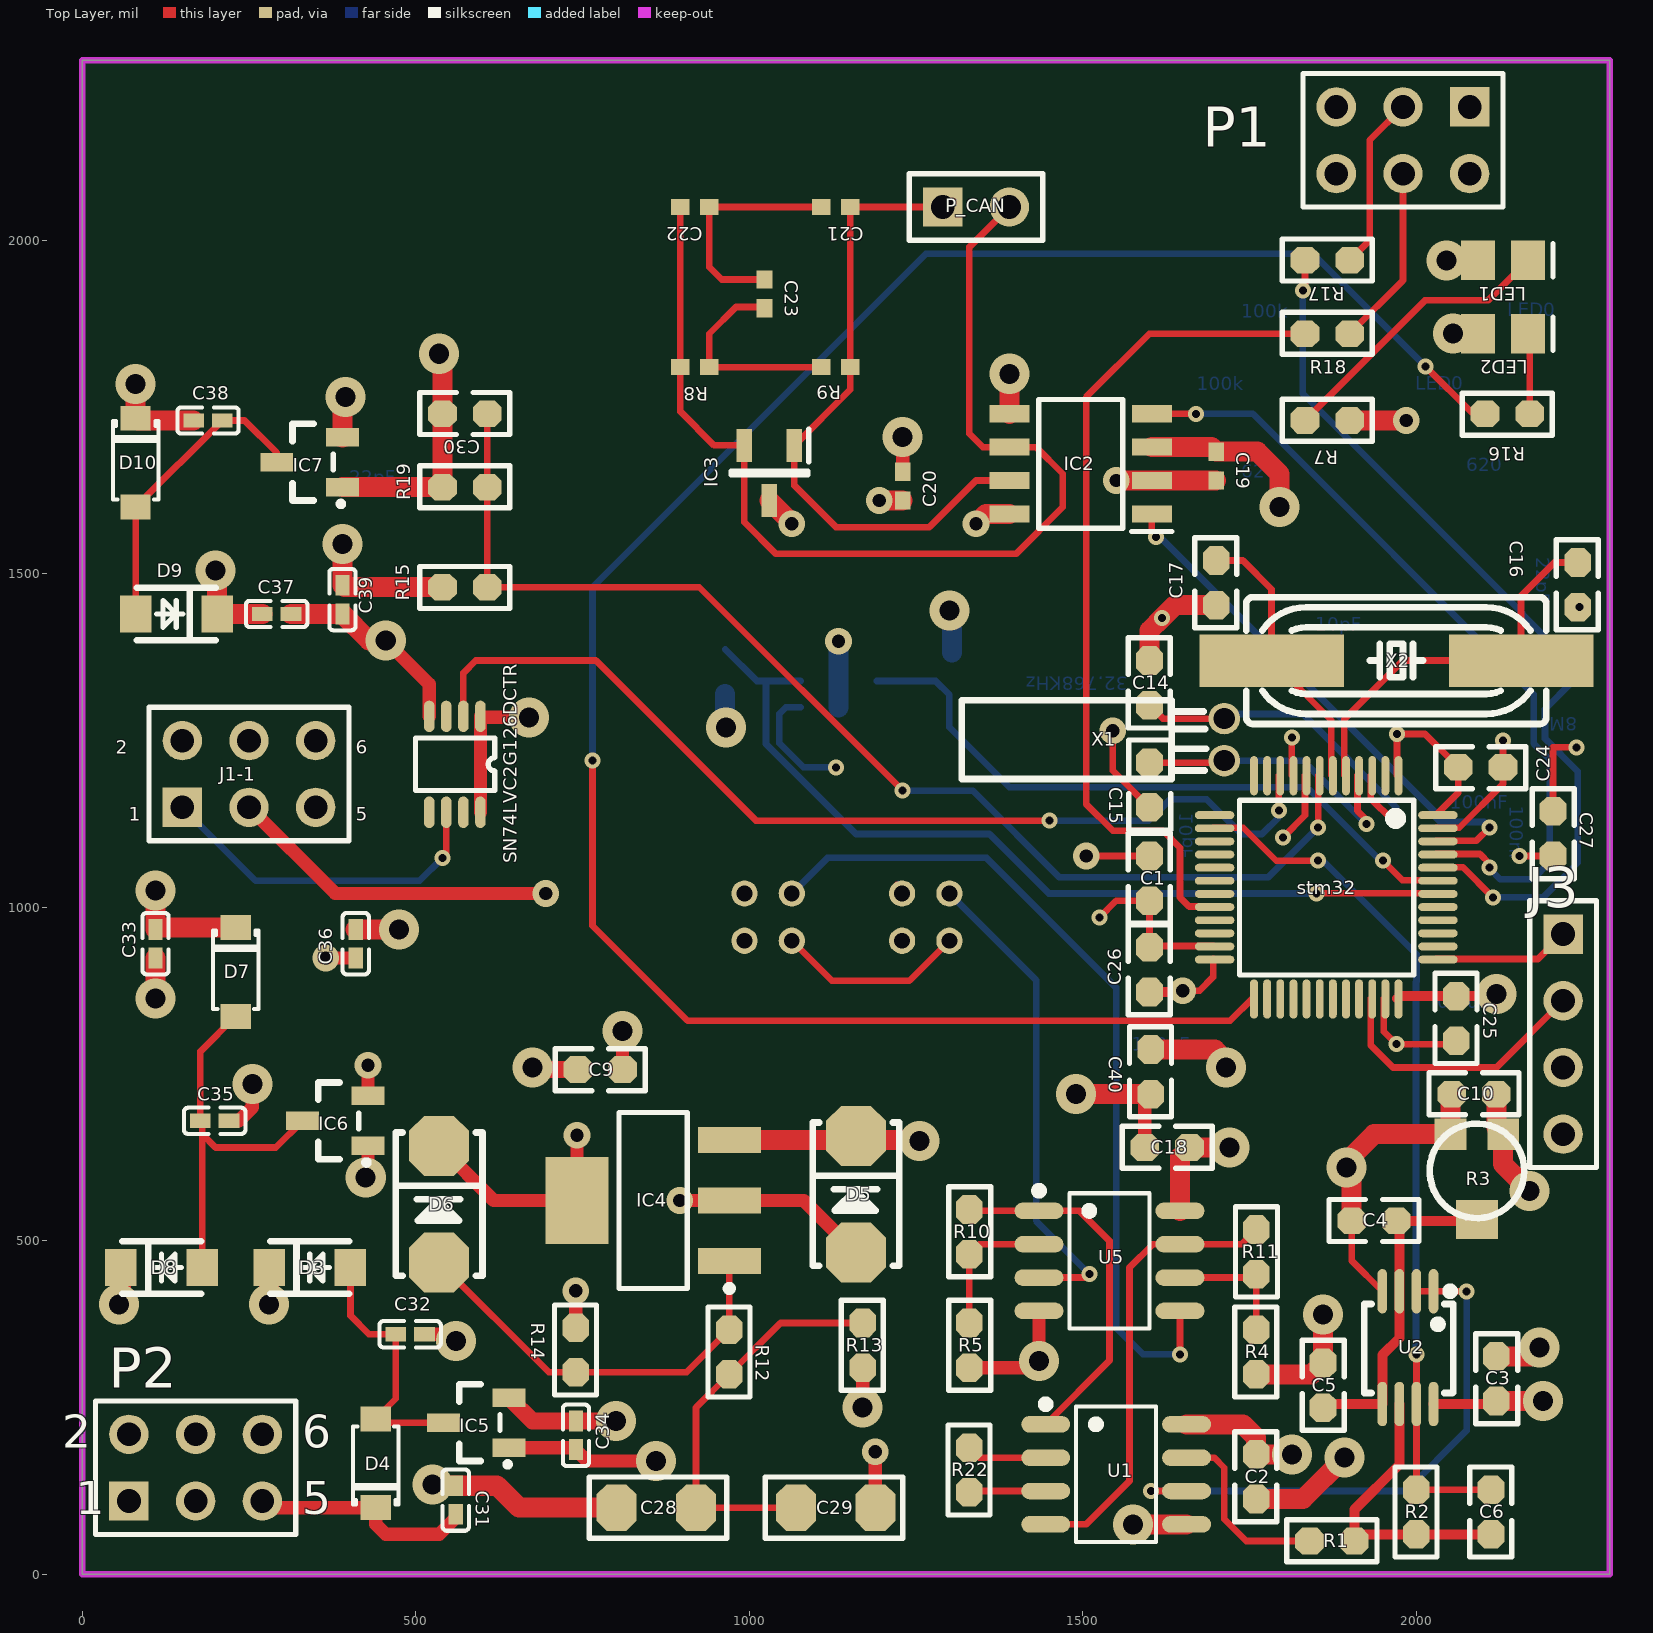
[diagram p0: Top Layer view]
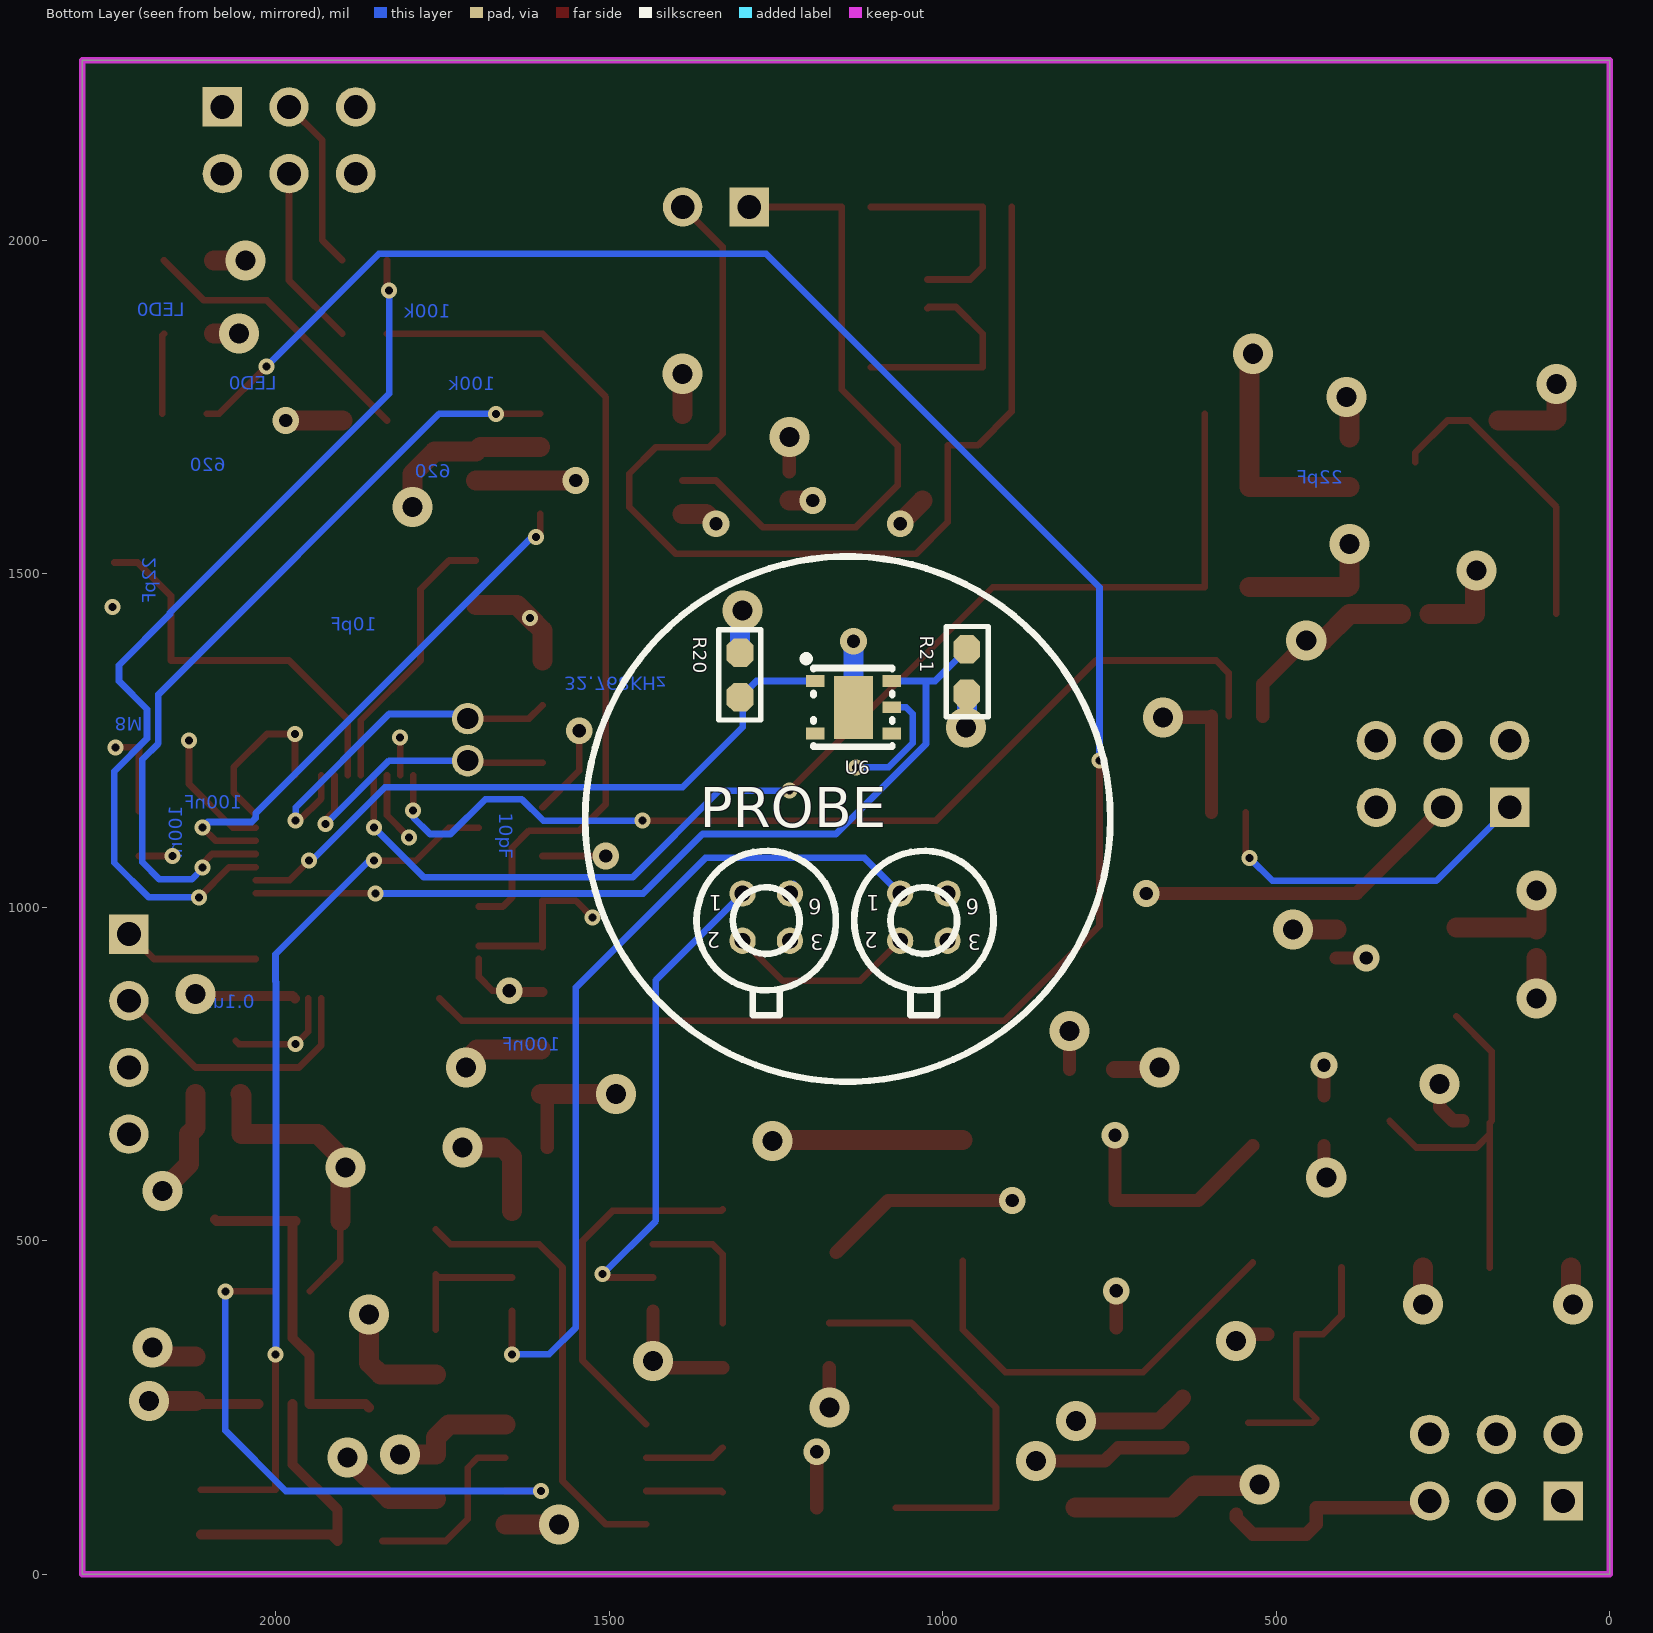
[diagram p1: Bottom Layer view, seen from below]
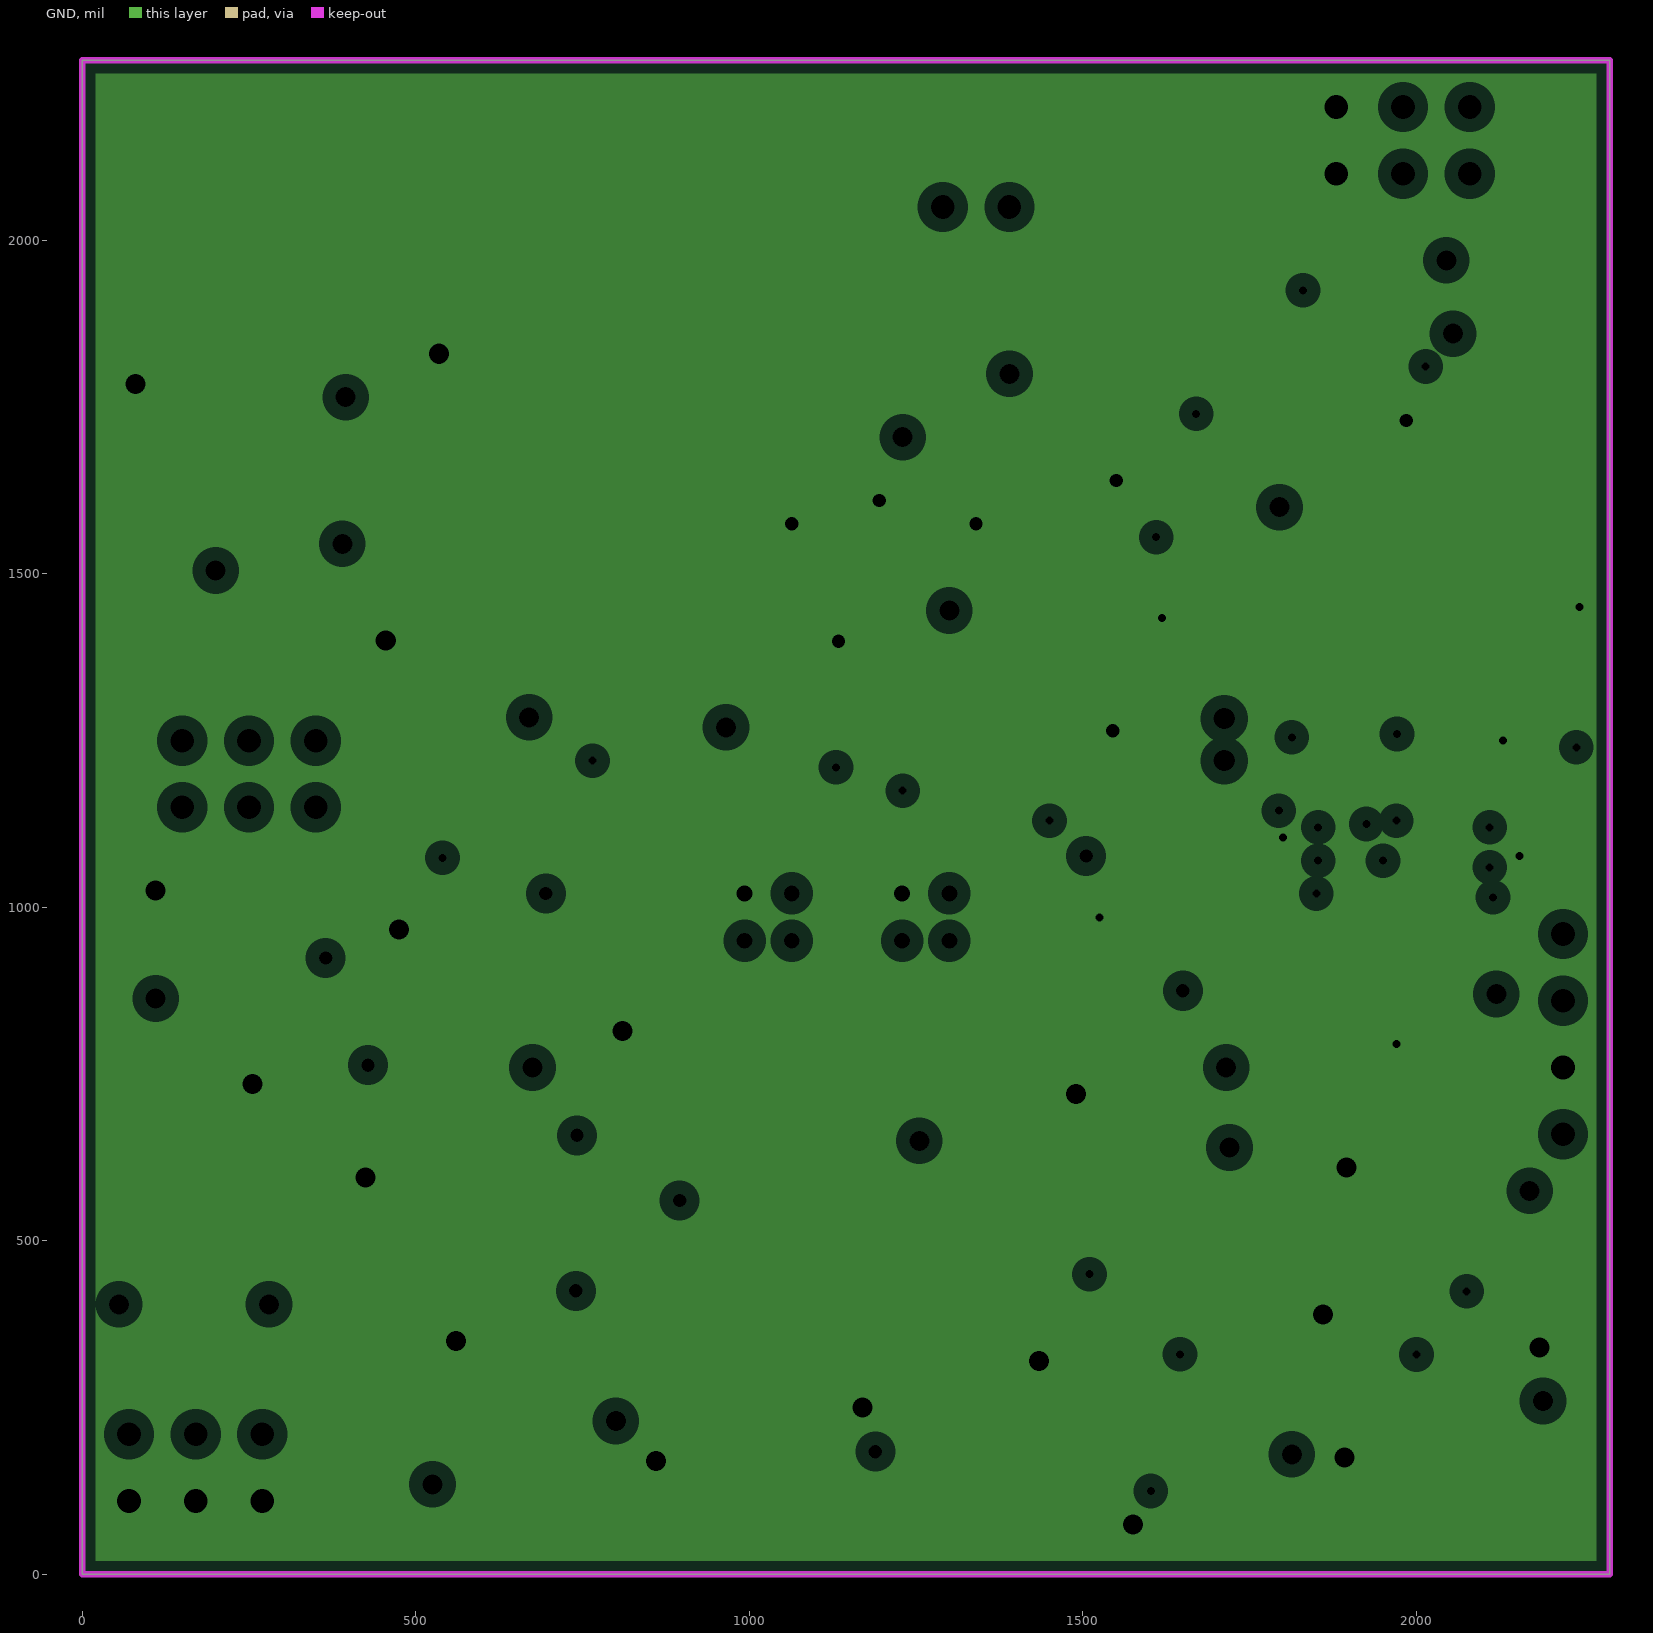
[diagram p2: GND, clearances drawn from the general rule]
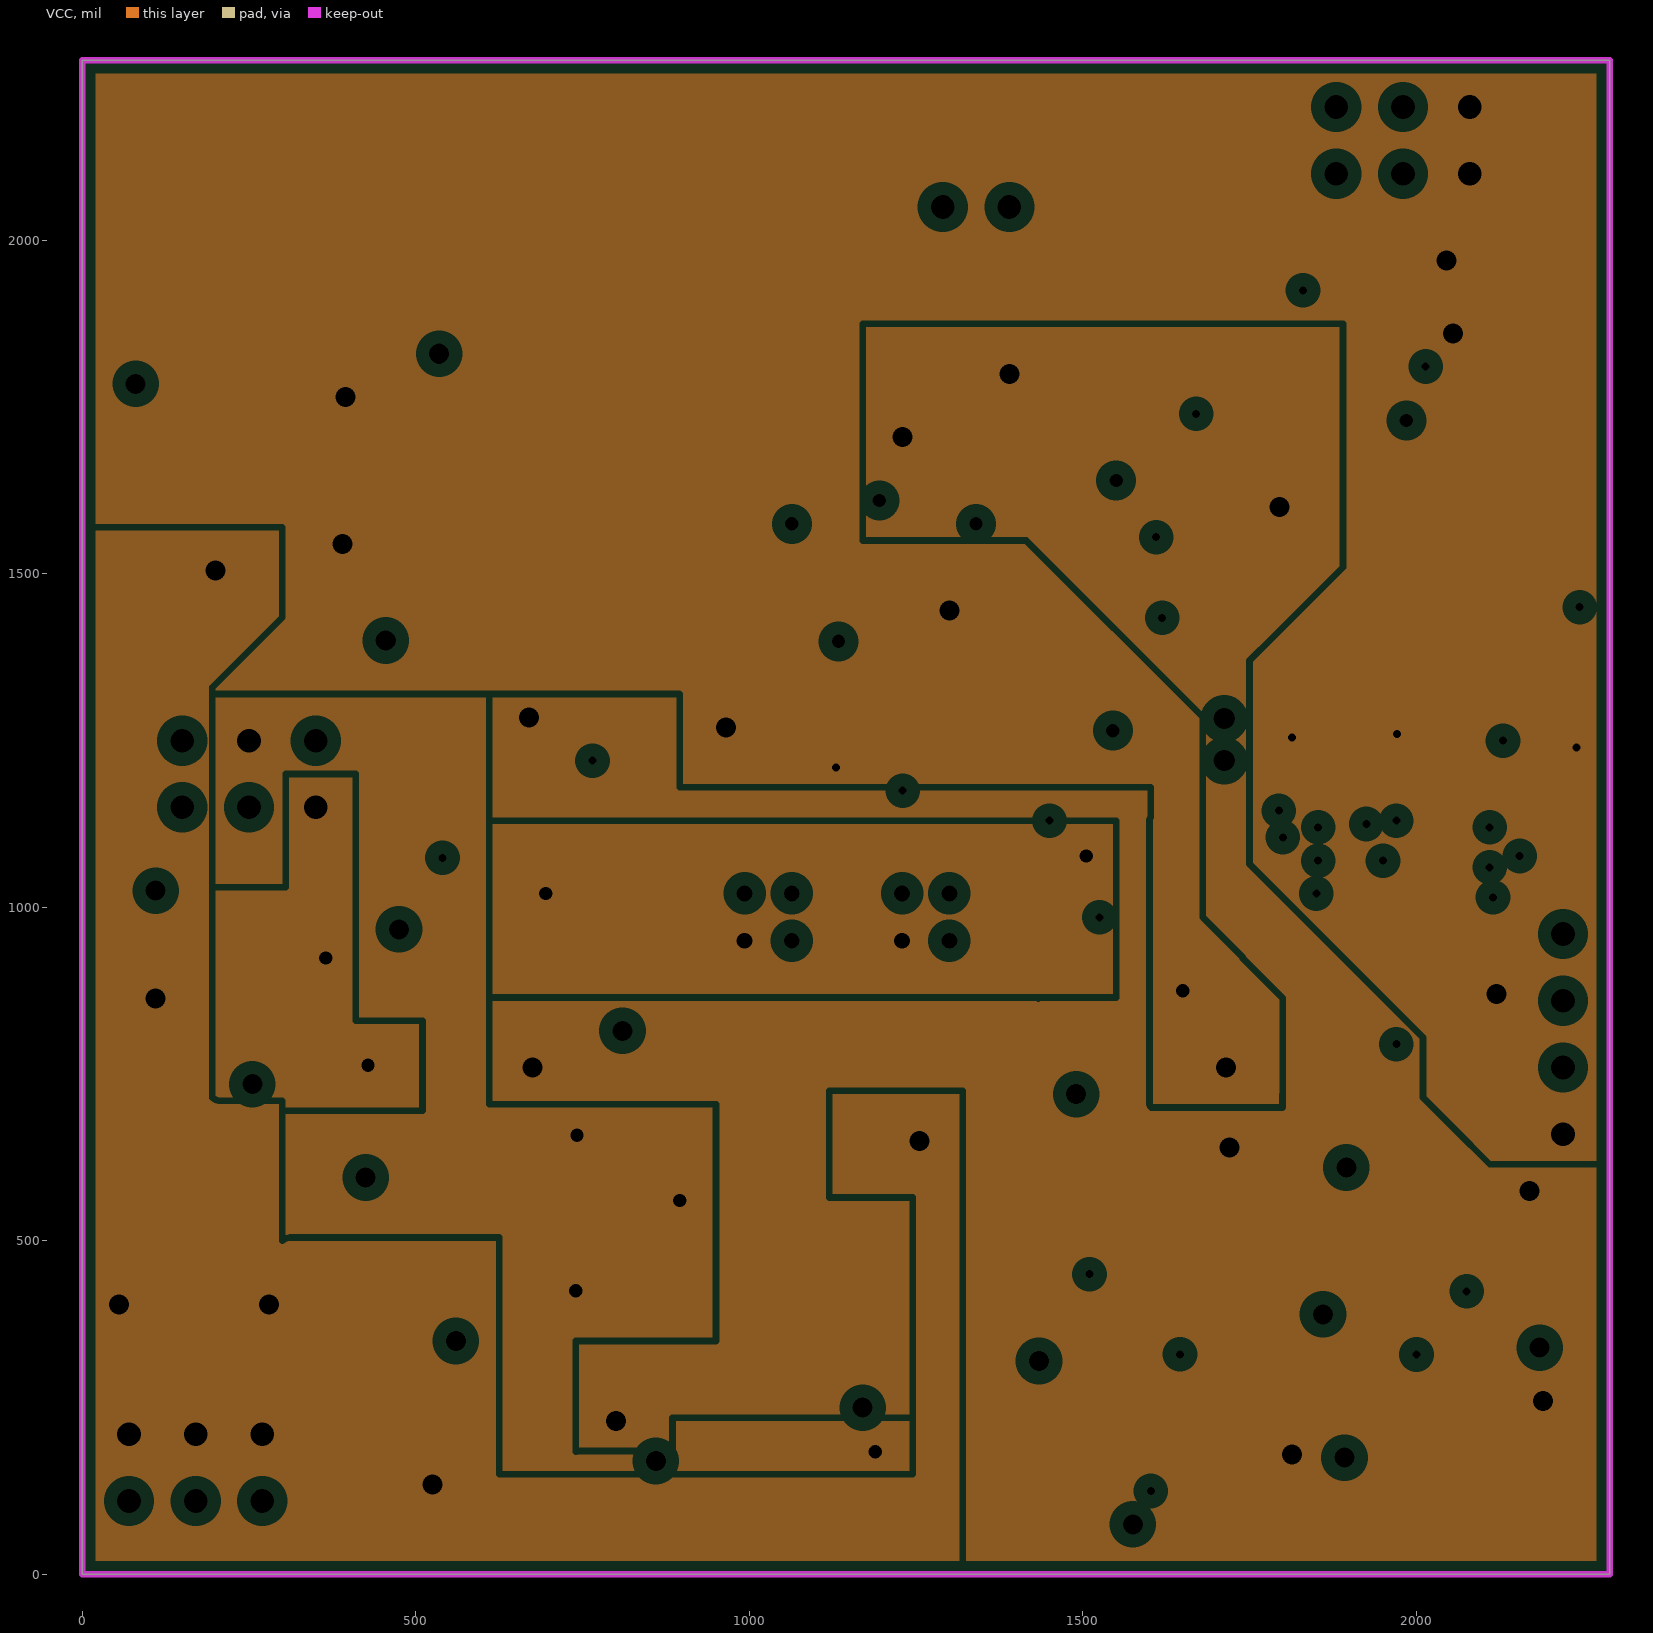
[diagram p3: VCC, clearances drawn from the general rule]
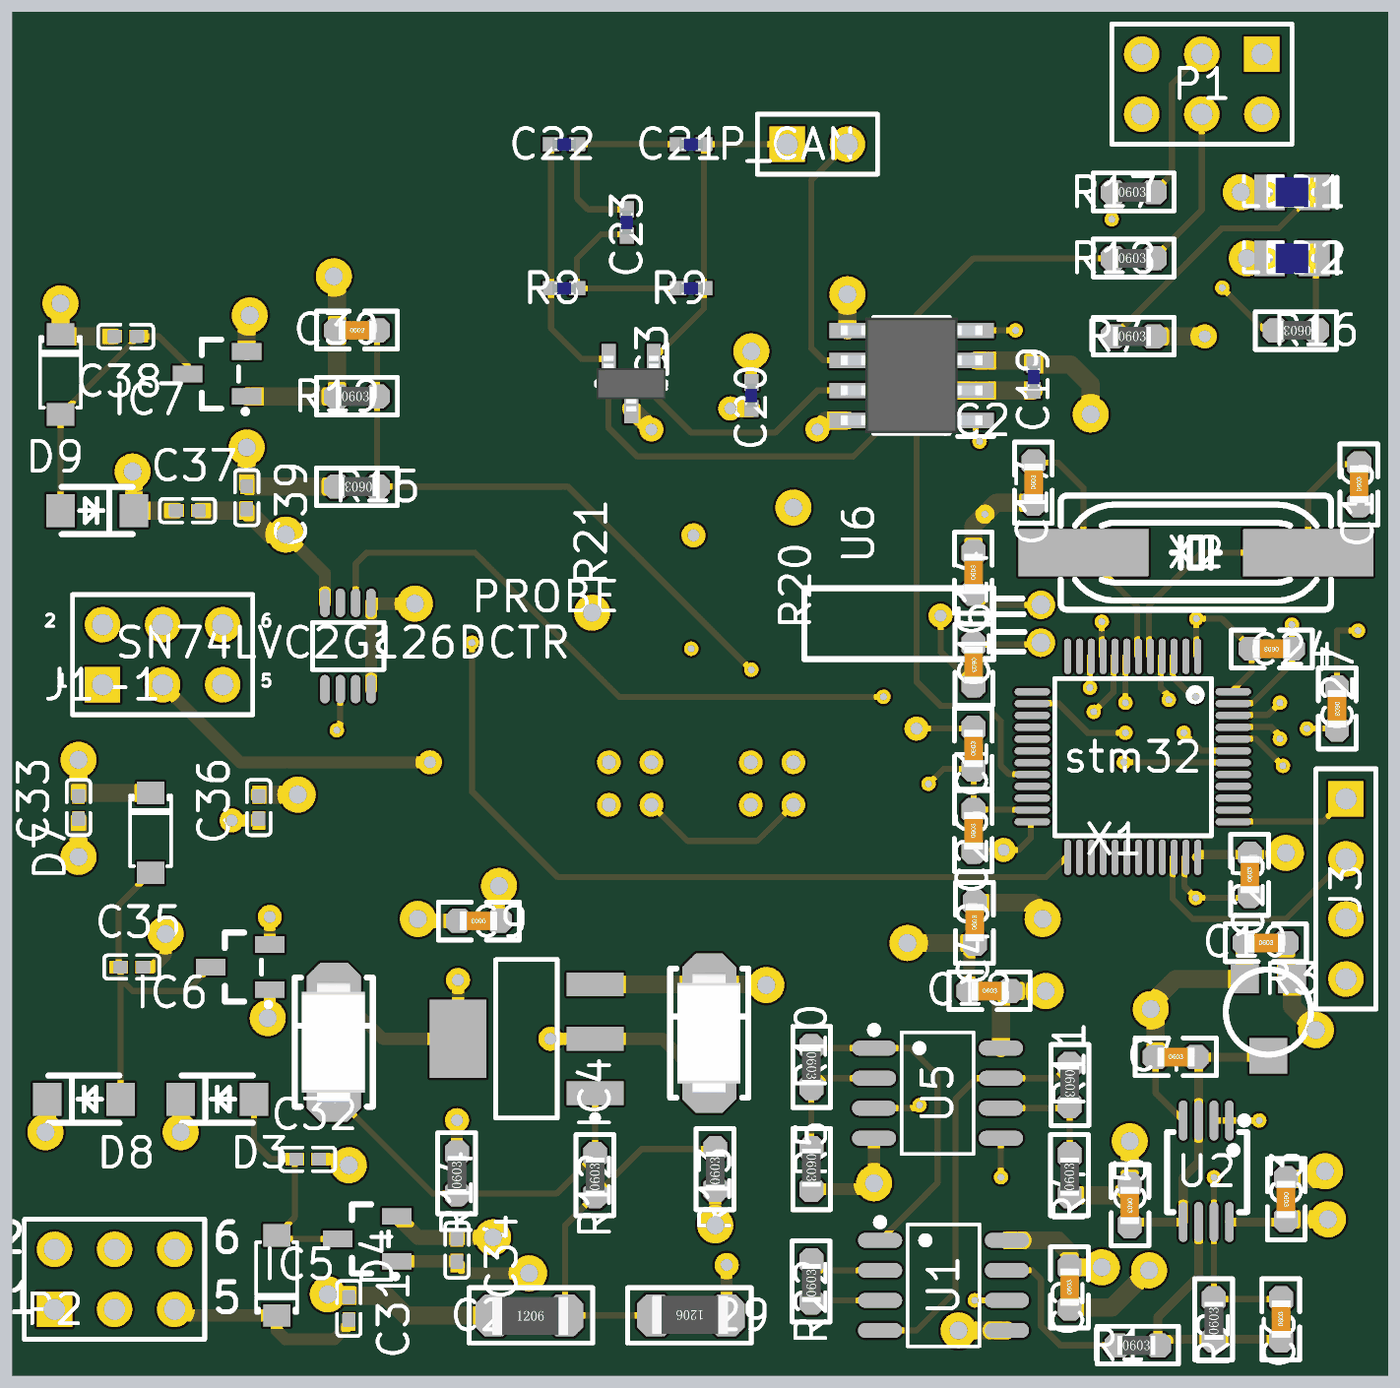
[diagram p4: 3D render of the assembled board from above, using the file's embedded part models]
# Altium PCB MISC82170.PcbDoc (part 1 of 2)
Units mil, origin at the board's own origin, x right, y up, seen from the top; angles counter-clockwise.
Board outline 2290 x 2270 mil, 4 copper layers (Top Layer, GND, VCC, Bottom Layer), stack 43.156 mil thick; 86 components, 73 nets, 279 pads, 92 vias.

## Layer stack, top to bottom
Top Solder: solder mask 0.4, Solder Resist, Dk 3.5
Top Layer: signal copper 1.4
Dielectric1: core 10, FR-4, Dk 4.2
Dielectric4: dielectric 12.6, FR-4, Dk 4.8
GND: plane copper 1.378, net GND
Dielectric 2: prepreg 5, Dk 4.2
VCC: plane copper 1.378
Dielectric 2: core 10, Dk 4.2
Bottom Layer: signal copper 1.4
Bottom Solder: solder mask 0.4, Solder Resist, Dk 3.5

## Board outline
0,30 0,2270 2290,2270 2290,0 0,0

## Design rules (kind name [scope] priority, off if disabled: settings)
Clearance [All] p1: gap=0
ComponentClearance [All] p1: gap=0 collisioncheckmode=3 verticalgap=10 showdistances=FALSE
FabricationTestpoint [(IsPad And (OnTopLayer Or OnBottomLayer))] p1: side=3 testpointundercomponent=TRUE minsize=40 maxsize=100 preferedsize=60 minholesize=0 maxholesize=40 preferedholesize=32 testpointgrid=1 allowsidetop=TRUE allowsidebottom=TRUE usegrid=TRUE gridtolerance=0.01
HoleToHoleClearance [All] p1: gap=0 allowstackedmicrovias=TRUE
MinimumSolderMaskSliver [All] p1: minsoldermaskwidth=0
PlaneClearance [All] p1: clearance=20
PlaneConnect [All] p1: planeconnectstyle=Relief reliefexpansion=20 reliefentries=4 reliefconductorwidth=10 reliefairgap=10
PolygonConnect [All] p1: connectstyle=Relief reliefconductorwidth=10 reliefentries=4 polygonreliefangle="90 Angle" airgapwidth=10
RoutingVias [All] p1: holewidth=28 width=50 viastyle="Through Hole" minholewidth=12 minwidth=24 maxholewidth=12 maxwidth=24
SilkToSilkClearance [All] p1: silktosilkclearance=0
SilkToSolderMaskClearance [IsPad] p1: minsilkscreentomaskgap=0 clearancetoexposedcopper=TRUE
SolderMaskExpansion [All] p1: expansion=4
Width [All] p1: maxlimit=30 minlimit=10 preferedwidth=10 minimp=50.000000 maximp=50.000000 favimp=50.000000
22 further rules are at their usual default settings.

## Components (designator, comment, footprint, x,y, rotation, side; value= is the part's Value field where it differs from the comment)
C1 "Cap" C_C0603_M 1598,1010 r90 top
C2 "Cap" C_C0603_M 1758,113 r90 top
C3 "Cap" C_C0603_M 2122,327 r270 top
C4 "Cap" C_C0603_M 1903,532 r0 top
C5 "0.1uF" C_C0603_M 1862,317 r270 top
C6 "Cap" C_C0603_M 2110,60 r90 top
C9 "Cap" C_C0603_M 810,755 r180 top
C10 "Cap" C_C0603_M 2053,722 r0 top
C14 "10pF" C_C0603_M 1598,1303 r90 top
C15 "10pF" C_C0603_M 1602,1217 r270 top
C16 "22pF" C_C0603_M 2240,1450 r90 top
C17 "22pF" C_C0603_M 1698,1453 r90 top
C18 "Cap" C_C0603_M 1593,642 r0 top
C19 "100nF" CAPC1005X37N 1700,1641.97 r90 top
C20 "100nF" CAPC1005X37N 1230,1611.97 r90 top
C21 "100pF" CAPC1005X37N 1110,2050 r0 top
C22 "100pF" CAPC1005X37N 898.66,2050 r0 top
C23 "4.7nF" CAPC1005X37N 1022.89,1900 r90 top
C24 "100nF" C_C0603_M 2130,1208 r180 top
C25 "0.1uF" C_C0603_M 2058,800 r90 top
C26 "100nF" C_C0603_M 1598,873 r90 top
C27 "100nF" C_C0603_M 2207,1144 r270 top
C28 "10uF" C_R1206 801,100 r0 top
C29 "10uF" C_R1206 1189,100 r180 top
C30 "1uF" C_C0603_M 540,1742 r0 top
C31 "Cap0402" C0402 634.63,100.45 r90 top
C32 "Cap0402" C0402 502.47,434.63 r180 top
C33 "Cap0402" C0402 35.37,956.55 r270 top
C34 "Cap0402" C0402 814.63,197.53 r90 top
C35 "Cap0402" C0402 209.55,754.63 r180 top
C36 "Cap0402" C0402 335.37,956.55 r270 top
C37 "Cap0402" C0402 302.47,1514.63 r180 top
C38 "Cap0402" C0402 177.53,1655.37 r0 top
C39 "Cap0402" C0402 464.63,1450.45 r90 top
C40 "Cap" C_C0603_M 1600,720 r90 top
D3 "GS1004FL" GS1004FL 411.38,370.63 r0 top
D4 "PTVS36VS1UTR" PTVS36VS1UTR 607.79,196.3 r90 top
D5 "IN4007" C_DO-214AC 1160,570 r270 top
D6 "IN4007" C_DO-214AC 535,555 r270 top
D7 "PTVS36VS1UTR" PTVS36VS1UTR 62.21,873.7 r270 top
D8 "GS1004FL" GS1004FL 189.33,370.63 r0 top
D9 "GS1004FL" GS1004FL 70.67,1529.37 r180 top
D10 "PTVS36VS1UTR" PTVS36VS1UTR -87.79,1636.96 r270 top
IC2 "TJA1051T_1J" SOIC-8 1601.77,1590 r180 top
IC3 "NUP2105LT1G" SOT-23A-3 1065,1691.34 r270 top
IC4 "LM317DCY" SOT223A 970,470 r90 top
IC5 "MCP1792T-5002H_CB" MCP1792T-220 476.98,185 r0 top
IC6 "MCP1792T-2.2V" MCP1792T-220 265.38,637.6 r0 top
IC7 "MCP1792T-3.3V" MCP1792T-220 226.98,1625 r0 top
J1-1 "source_select" HDR2X3 150,1150 r0 top
J3 "SW debug pin" HDR4X1_A 2220,810 r270 top
LED1 "LED0" LED_0805_Blue 2130,1970 r0 top
LED2 "LED0" LED_0805_Blue 2130,1860 r0 top
P1 "Header 3*2" HDR3X2 1980,2150 r180 top
P2 "Header 3X2" HDR2X3 70,110 r0 top
P_CAN "Header 2" HDR1X2 1290,2050 r0 top
PROBE "Header 4X2" PROBE 887.24,1296.65 r0 bottom
R1 "10K" C_R0603 1840,50 r0 top
R2 "24.9K" C_R0603 2000,60 r90 top
R3 "100K" VG039N 2130,660 r180 top
R4 "10K" C_R0603 1760,300 r90 top
R5 "10K" C_R0603 1330,377 r270 top
R7 "620" C_R0603 1833,1730 r0 top
R8 "62R" R0402 898.66,1810 r0 top
R9 "62R" R0402 1110,1810 r0 top
R10 "30K" C_R0603 1330,547 r270 top
R11 "30K" C_R0603 1760,517 r270 top
R12 "13K" C_R0603 970,300 r90 top
R13 "300" C_R0603 1170,310 r90 top
R14 "25.5k" C_R0603 740,303 r90 top
R15 "10K" C_R0603 607,1480 r180 top
R16 "620" C_R0603 2170,1740 r180 top
R17 "100k" C_R0603 1833,1970 r0 top
R18 "100k" C_R0603 1833,1860 r0 top
R19 "0R" C_R0603 540,1630 r0 top
R20 "4.7K" C_R0603 1303.78,1314.97 r90 bottom
R21 "4.7K" C_R0603 963.78,1387 r270 bottom
R22 "953R" C_R0603 1330,123 r90 top
SN74LVC2G126DCTR "SN74LVC2G126DCTR" SN74LVC2G126DCTR1 550,1220 r180 top
stm32 "STM32F103C8T6" STM32F103C8T6 1865,1030 r180 top
U1 "AD8422ARZ" AD8422ARZ 1550,150 r270 top
U2 "ADA4096-2ARMZ" ADA4096-2ARMZ 1987.4,340 r180 top
U5 "AD8539ARZ" AD8422ARZ 1540,470 r270 top
U6 "HTU21D" htu21d 1408.6,1401.77 r270 bottom
X1 "32.768KHz" 直插晶振-32.768khz 1833.37,892.46 r0 top
X2 "8M" HC-49S_L11.4-W4.8-8HZ 1970,1370 r180 top

## Footprints (in the part's own frame and the unit in brackets; to place one, negate y for a bottom-side part, rotate by r counter-clockwise, add the part's x,y. Pads: shape width x height; smd on the part's side, far side on the other; paste and mask are expansions set on the pad)
AD8422ARZ [mm]
  oval 0.63x1.865 smd: 1(-1.905,-2.682) 2(-0.635,-2.682) 3(0.635,-2.682) 4(1.905,-2.682) 5(1.905,2.682) 6(0.635,2.682) 7(-0.635,2.682) 8(-1.905,2.682)
  silkscreen extent -2.82,-2.83 2.58,1.52
ADA4096-2ARMZ [mil]
  oval 14.33x66.61 smd: 1(-38.39,-84.49) 2(-12.79,-84.49) 3(12.8,-84.49) 4(38.39,-84.49) 5(38.39,84.49) 6(12.8,84.49) 7(-12.79,84.49) 8(-38.39,84.49)
  silkscreen extent -69,-90 65,68
C0402 [mm]
  rect 0.79x0.54 smd paste-100 mask+0.051: 1(-0.265,1.896) 2(0.825,1.896)
  silkscreen extent -0.89,1.4 1.45,2.39
C_C0603_M [mil]
  oct 43x40 smd: 1(0,-2) 2(67,-2)
  silkscreen extent -34,-33 101,30, body extent 3,-18 66,14, height 32
C_DO-214AC [mil]
  oct 90x90 smd: 1(87.5,0) 2(-87.5,0)
  silkscreen extent -108,-65 108,65, body extent -100,-53 100,52, height 84
C_R0603 [mil]
  oct 43x40 smd: 1(0,0) 2(67,0)
  silkscreen extent -34,-31 101,32, body extent 0,-16 63,16, height 18
C_R1206 [mil]
  oct 60x70 smd: 1(0,0) 2(119,0)
  silkscreen extent -41,-46 165,46, body extent -2,-32 124,31, height 24
CAPC1005X37N [mm]
  rect 0.7x0.6 smd: 1(-0.05,0) 2(1.05,0)
  body extent 0,-0.25 1,0.25, height 0.32
GS1004FL [mm]
  rect 1.2x1.4 smd: 1(-3.337,2.27) 2(-0.237,2.27)
  silkscreen extent -3.29,1.27 -0.29,3.27
HC-49S_L11.4-W4.8-8HZ [mm]
  rect 5.5x2 smd paste+0 mask+0.102: 1(-4.75,0) 2(4.75,0)
  silkscreen extent -5.71,-2.41 5.71,2.41
HDR1X2 [mm] "Connector; Header; 2 Position"
  rect 1.5x1.5 hole 0.9: 1(0,0)
  round 1.5 hole 0.9: 2(2.54,0)
  silkscreen extent -1.27,-1.27 3.81,1.27
HDR2X3 [mm] "Connector; Header; 3x2 Position"
  rect 1.5x1.5 hole 0.9: 1(0,0)
  round 1.5 hole 0.9: 2(0,2.54) 3(2.54,0) 4(2.54,2.54) 5(5.08,0) 6(5.08,2.54)
  silkscreen extent -1.27,-1.27 6.35,3.81
HDR3X2 [mm]
  rect 1.5x1.5 hole 0.9: 1(-2.54,-1.27)
  round 1.5 hole 0.9: 2(-2.54,1.27) 3(0,-1.27) 4(0,1.27) 5(2.54,-1.27) 6(2.54,1.27)
  silkscreen extent -3.81,-2.54 3.81,2.54, body extent -3.81,-2.54 3.81,2.54, height 8.57
HDR4X1_A [mm]
  rect 1.5x1.5 hole 0.9: 1(-3.81,0)
  round 1.5 hole 0.9: 2(-1.27,0) 3(1.27,0) 4(3.81,0)
  silkscreen extent -5.08,-1.27 5.08,1.27, body extent -5.08,-1.27 5.08,1.27, height 8.57
htu21d [mm]
  rect 0.45x0.701 smd: 1(1.585,5.53) 3(3.585,5.53) 4(3.585,8.431) 5(2.585,8.431) 6(1.585,8.431)
  rect 2.4x1.5 smd: 7(2.585,6.98)
  silkscreen extent 0.64,5.08 4.09,8.45
LED_0805_Blue [mm]
  rect 1.3x1.5 smd: 1(-0.95,0) 2(0.95,0)
  silkscreen extent 1.91,-0.64 1.91,0.64, body extent -1,-0.63 1,0.62, height 1.1
MCP1792T-220 [mm]
  rect 1.25x0.7 smd: 1(4.141,0.127) 2(4.141,2.027) 3(1.641,1.077)
  silkscreen extent 2.24,-0.61 4.18,2.54
PROBE [mm]
  round 1 hole 0.6: 1(4.484,7.005) 2(4.484,8.805) 3(2.684,8.805) 4(2.684,7.005) 5(10.484,7.005) 6(10.484,8.805) 7(8.684,8.805) 8(8.684,7.005)
  Top Layer lines w0.254: 2.656,6.797 2.721,6.732 ; 2.827,8.711 2.864,8.675 ; 4.444,6.732 4.484,6.732 4.521,6.732 ; 8.406,8.689 8.487,8.608 ; 8.548,8.546 8.487,8.608 ; 8.548,6.746 8.548,6.645 ; 8.487,8.608 8.487,8.608
  Bottom Layer lines w0.254: 4.521,8.532 4.639,8.65 4.643,8.654 ; 8.479,6.677 8.548,6.746
  silkscreen extent 0.93,5.38 12.24,11.64
PTVS36VS1UTR [mm]
  rect 0.95x1.15 smd: 1(-2.446,4.262) 2(0.939,4.262)
  silkscreen extent -2.33,3.4 0.65,5.13
R0402 [mm]
  rect 0.7x0.6 smd: 1(-0.05,0) 2(1.05,0)
  body extent 0,-0.25 1,0.25, height 0.32
SN74LVC2G126DCTR1 [mm]
  oval 0.4x1.2 smd: 1(-1.193,-1.686) 2(-0.543,-1.686) 3(0.107,-1.686) 4(0.757,-1.686) 5(0.757,1.964) 6(0.107,1.964) 7(-0.543,1.964) 8(-1.193,1.964)
  silkscreen extent -1.74,-0.86 1.28,1.14
SOIC-8 [mm]
  rect 1.525x0.65 smd: 1(-0.045,0) 2(-0.045,-1.27) 3(-0.045,-2.54) 4(-0.045,-3.81) 5(5.379,-3.81) 6(5.379,-2.54) 7(5.379,-1.27) 8(5.379,0)
  silkscreen extent -0.81,-4.35 4.27,0.67, body extent -0.33,-4.36 5.67,0.55, height 1.75
SOT223A [mm] "SOT223, 4-Leads, Body 6.7x7.3mm (max), Pitch 2.30mm, IPC Medium Density"
  rect 1x2.4 smd: 1(0,0) 2(2.3,0) 3(4.6,0)
  rect 3.3x2.4 smd: 4(2.3,5.8)
  silkscreen extent -1.17,-0.13 5.65,4.2, body extent -1.05,1.04 5.65,4.75, height 1.8
SOT-23A-3 [mm]
  rect 1.25x0.6 smd: 1(-0.034,0.066) 2(-0.034,-1.844) 3(2.066,-0.889)
  silkscreen extent -0.66,-2.35 1.09,0.62, body extent -0.17,-2.35 2.2,0.57, height 1.11
STM32F103C8T6 [mm]
  oval 0.3x1.5 smd paste+0 mask+0.102: 1(-2.75,-4.25) 2(-2.25,-4.25) 3(-1.75,-4.25) 4(-1.25,-4.25) 5(-0.75,-4.25) 6(-0.25,-4.25) 7(0.25,-4.25) 8(0.75,-4.25) 9(1.25,-4.25) 10(1.75,-4.25) 11(2.25,-4.25) 12(2.75,-4.25) 25(2.75,4.25) 26(2.25,4.25) 27(1.75,4.25) 28(1.25,4.25) 29(0.75,4.25) 30(0.25,4.25) 31(-0.25,4.25) 32(-0.75,4.25) 33(-1.25,4.25) 34(-1.75,4.25) 35(-2.25,4.25) 36(-2.75,4.25)
  oval 1.5x0.3 smd paste+0 mask+0.102: 13(4.25,-2.75) 14(4.25,-2.25) 15(4.25,-1.75) 16(4.25,-1.25) 17(4.25,-0.75) 18(4.25,-0.25) 19(4.25,0.25) 20(4.25,0.75) 21(4.25,1.25) 22(4.25,1.75) 23(4.25,2.25) 24(4.25,2.75) 37(-4.25,2.75) 38(-4.25,2.25) 39(-4.25,1.75) 40(-4.25,1.25) 41(-4.25,0.75) 42(-4.25,0.25) 43(-4.25,-0.25) 44(-4.25,-0.75) 45(-4.25,-1.25) 46(-4.25,-1.75) 47(-4.25,-2.25) 48(-4.25,-2.75)
  silkscreen extent -3.33,-3.31 3.3,3.34
VG039N [mm]
  rect 1.2x1.2 smd: 1(2,0) 3(0,0)
  rect 1.6x1.5 smd: 2(1,3.25)
  silkscreen extent -0.81,-0.4 2.79,3.2
直插晶振-32.768khz [mm]
  round 1.2 hole 0.8: 1(-3.081,9.92) 2(-3.081,8.32)
  silkscreen extent -13.08,7.62 -3.78,10.62

## Part data
C1 C2 C3 C4 C6 C9 C10 C18 C31 C32 C33 C34 C35 C36 C37 C38 C39 C40: "Capacitor"
C5: library part Cap, "Capacitor"
C19 C20 C21 C22 C23: library part Cap0402, "Capacitor"
C25: library part 1uF
C28 C29: library part CAP
D3 D8 D9: library part 1N4148, "Diode"
D4 D7 D10: library part TVS
D5 D6: library part Diode, "Default Diode"
IC2 IC3: "Integrated Circuit"
IC5 IC6 IC7: library part MCP1792T-3302H_CB, "Integrated Circuit"
J1-1: library part "Header 3X2", "Header, 3-Pin, Dual row"
J3: library part "Header 4", "Connector"
LED1 LED2: "Light-emitting diode"
P1: "Connector"
P2: "Header, 3-Pin, Dual row"
P_CAN: "Header, 2-Pin"
PROBE: "Header, 4-Pin, Dual row"
R1 R2 R4 R5 R10 R11 R20 R21 R22: library part Res1, "Resistor"
R3: library part "RPot SM", "Square Trimming Potentiometer"
R8 R9: library part Res0402, "Resistor"
R12 R13 R14: library part SR_110K0603±1%_VISHAY, "Resistor"
R17 R18: library part 620
R19: library part 10K
X1 X2: library part XTAL, "Crystal oscillator"

## Via types
v1: diameter 60, hole 30, Top Layer to Bottom Layer, 42 vias
v2: diameter 24, hole 12, Top Layer to Bottom Layer, 34 vias
v3: diameter 40, hole 20, Top Layer to Bottom Layer, 16 vias

## Nets (pads, with @x,y where several pads share a name; then routed paths per layer and width w, separated by ;. In a path a pad name is that pad's centre, name@x,y a point inside that pad or via, vN(x,y) a via of type N, cw(c..) or ccw(c..) an arc to the next point about the centre after c; other vN are vias at no path point)
1Yinput: J1-1.1 SN74LVC2G126DCTR.6 | length 524
  Top Layer w10: v2(540,1074.22) 545.78,1074.22 SN74LVC2G126DCTR.6@545.78,1142.68
  Bottom Layer w10: J1-1.1@150,1150 260,1040 505.78,1040 v2(540,1074.22)
2Vinput: C36.2 IC6.2 J1-1.5 | length 91
  Top Layer w20: v3(365,924.08) C36.2@410,924.08 ; IC6.2@428.4,717.4 v3(428.4,763.4)
2Vinput-2: C29.1 D5.1 D6.2 IC4.2 IC4.4 J1-1.4 R14.2 | length 774.2
  Top Layer w20: D6.2@535,642.5 616.95,560.55 IC4.4@741.65,560.55 v3(741.65,658.35) ; R14.2@740,370 v3(740,425) ; v3(895.55,560.55) IC4.2@970,560.55 1081.95,560.55 D5.1@1160,482.5 ; C29.1@1189,100 v3(1189,184)
5V: C2.2 C3.2 C9.2 C10.2 C18.2 C19.2 C20.2 C34.2 IC2.3 IC2.5 IC5.2 R3.3 SN74LVC2G126DCTR.1 SN74LVC2G126DCTR.8 U1.8 U2.8 U5.8 | length 1514.6
  Top Layer w15: U2.8@2025.79,255.51 2115.51,255.51 C3.2@2120,260
  Top Layer w20: SN74LVC2G126DCTR.8@596.97,1142.68 SN74LVC2G126DCTR.1@596.97,1286.38 598.35,1285 v1(670,1285) ; C20.2@1230,1653.31 v1(1230,1705)
  Top Layer w25: IC5.2@640,264.8 674.8,230 C34.2@740,230 v1(800,230) ; v1(675,760) 678,757 C9.2@743,757
  Top Layer w30: IC2.5@1390,1740 v1(1390,1800) ; IC2.3@1603.54,1690 1693.31,1690 C19.2@1700,1683.31 1761.69,1683.31 1795,1650 v1(1795,1600) ; U5.8@1645.61,545 1645.61,625.61 C18.2@1660,640 v1(1720,640) ; U1.8@1655.61,225 1740,225 1760,205 C2.2@1760,180 v1(1813.46,180) ; C3.2@2120,260 v1(2190,260) ; C10.2@2120,720 2120,670 R3.3@2130,660 2130,615 v1(2170,575)
12V: C28.1 C31.2 C33.2 C37.2 D3.1 D5.2 D8.1 D9.1 IC4.3 P2.2 P2.4 P2.6 | length 881.6
  Top Layer w30: v1(55,405) 57.95,407.95 D8.1@57.95,460 ; v1(110,863.46) C33.2@110,924.08 ; v1(200,1505) 202.05,1502.95 D9.1@202.05,1440 C37.2@270,1440 ; v1(280,405) D3.1@280,460 ; v1(525,135) 527.08,132.92 C31.2@560,132.92 622.08,132.92 655,100 C28.1@801,100 ; IC4.3@970,651.1 1253.9,651.1 v1(1255,650)
BOOT0: R17.1 stm32.44 | length 1362.7
  Top Layer w10: v2(1830,1925) 1833,1928 R17.1@1833,1970 ; stm32.44@2030,1060.31 2069.69,1060.31 v2(2115,1015) v2@2115,1015.63
  Bottom Layer w10: v2(1830,1925) 1830,1770 2158.34,1441.66 2158.34,1439.62 2235,1362.95 2235,1339.17 2192.9,1297.07 2192.9,1252.94 2242,1203.83 2242,1067 2190,1015 v2(2115,1015)
CANH: C21.2 IC2.7 IC3.1 P_CAN.1 R9.2 | length 968.2
  Top Layer w10: P_CAN.1@1290,2050 C21.2@1151.34,2050 R9.2@1151.34,1810 1151.34,1776.42 IC3.1@1067.6,1692.68 1067.6,1632.4 1130,1570 1270,1570 1340,1640 IC2.7@1390,1640
CANL: C22.1 IC2.6 IC3.2 P_CAN.2 R8.1 | length 1644.5
  Top Layer w10: C22.1@896.69,2050 R8.1@896.69,1810 896.69,1743.31 947.32,1692.68 IC3.2@992.4,1692.68 992.4,1577.6 1040,1530 1400,1530 1470,1600 1470,1650 1430,1690 IC2.6@1390,1690 1350,1690 1330,1710 1330,1990 P_CAN.2@1390,2050
GND: C1.1 C2.1 C3.1 C4.1 C5.1 C9.1 C10.1 C14.2 C15.2 C16.1 C17.1 C18.1 C19.1 C20.1 C24.1 C25.1 C26.2 C27.2 C30.1 C31.1 C32.1 C33.1 C34.1 C35.1 C36.1 C37.1 C38.1 C39.1 C40.1 D4.1 D7.1 D10.1 IC2.2 IC2.8 IC3.3 IC5.1 IC6.1 IC7.1 J3.3 P1.5 P1.6 P2.1 P2.3 P2.5 PROBE.4 PROBE.8 R3.1 R4.1 R5.2 R7.2 R13.1 R19.1 SN74LVC2G126DCTR.4 stm32.8 stm32.23 stm32.35 stm32.47 U1.5 U2.4 U5.4 U6.7 | length 4766.1
  Top Layer w10: v2(1525,985) 1550,1010 C1.1@1600,1010 C26.2@1600,940 1602.2,942.2 stm32.23@1695.35,942.2 ; v3(1545,1265) 1545,1205 C15.2@1600,1150 ; v2(1800,1105) 1833.15,1138.15 stm32.8@1833.15,1198.11 ; C4.1@1903,530 1903,470.5 U2.4@1949.01,424.49 ; stm32.35@1951.26,863.46 1951.26,813.74 v2(1970,795) 2055,795 C25.1@2060,800 ; stm32.47@2030,1119.37 2064.37,1119.37 2130,1185 C24.1@2130,1210 v2(2130,1250) ; v2(2155,1077) C27.2@2205,1077 ; C16.1@2242,1450 v2(2245,1450)
  Top Layer w20: C35.1@220,680 235,680 255,700 v1(255,735) ; P2.5@270,110 280,100 D4.1@440,100 440,75 455,60 535,60 560,85 C31.1@560,90 ; v1(425,595) 428.4,598.4 IC6.1@428.4,642.6 ; v1(455,1400) 520.19,1334.81 SN74LVC2G126DCTR.4@520.19,1286.38 ; C32.1@512.92,360 550,360 v1(560,350) ; IC5.1@640,190 737.08,190 C34.1@740,187.08 757.08,170 v1(860,170) ; C9.1@810,757 v1(810,815) ; v1(1170,250) R13.1@1170,310 ; R5.2@1330,310 1424.39,310 v1(1434.39,320) U5.4@1434.39,395 ; C18.1@1593,640 1593,711 C40.1@1602,720
  Top Layer w30: v1(80,1785) D10.1@80,1733.26 83.26,1730 C38.1@167.08,1730 ; v1(110,1025) C33.1@110,967 113,970 D7.1@230,970 ; C37.1@312.92,1440 C39.1@390,1440 430,1400 v1(455,1400) ; IC7.1@390,1630 R19.1@540,1630 C30.1@540,1740 540,1825 v1(535,1830) ; C36.1@410,967 v1(475,967) ; IC3.3@1030,1610 1063.78,1576.22 v3(1063.78,1575) ; v3(1195,1610) C20.1@1230,1610 ; v3(1340,1575) 1355,1590 IC2.8@1390,1590 ; v1(1490,720) C40.1@1602,720 ; v3(1550,1640) IC2.2@1603.54,1640 C19.1@1700,1640 ; v1(1575,75) U1.5@1655.61,75 ; C14.2@1600,1370 1600,1415 v2(1619,1434) 1638,1453 C17.1@1700,1453 ; C2.1@1760,113 1830.21,113 v1(1892.21,175) ; R4.1@1760,300 1843,300 C5.1@1860,317 v1(1860,390) ; R7.2@1900,1730 v3(1985,1730) ; C4.1@1903,530 1903,602 v1(1895,610) 1895,618.42 1936.58,660 R3.1@2051.26,660 2051.26,718.26 C10.1@2053,720 ; C3.1@2120,327 2172,327 v1(2185,340)
  Bottom Layer w30: U6.7@1133.78,1300 v3(1133.78,1398.78) v3@1135,1400
NetC4_2: C4.2 C5.2 R3.2 U2.3 U2.5 | length 499.8
  Top Layer w15: C5.2@1860,250 1865.51,255.51 U2.5@1949.01,255.51 1949.01,329.01 1974.6,354.6 U2.3@1974.6,424.49 1974.6,525.4 C4.2@1970,530 2088.58,530 R3.2@2090.63,532.05
NetC6_1: C6.1 R1.2 R2.1 U2.6 | length 442.7
  Top Layer w15: U2.6@1974.6,255.51 1974.6,164.6 1907,97 R1.2@1907,50 1917,60 R2.1@2000,60 C6.1@2112,60
NetC21_1: C21.1 C22.2 C23.2 | length 348.7
  Top Layer w10: C23.2@1022.89,1941.34 958.66,1941.34 940,1960 C22.2@940,2050 C21.1@1108.03,2050